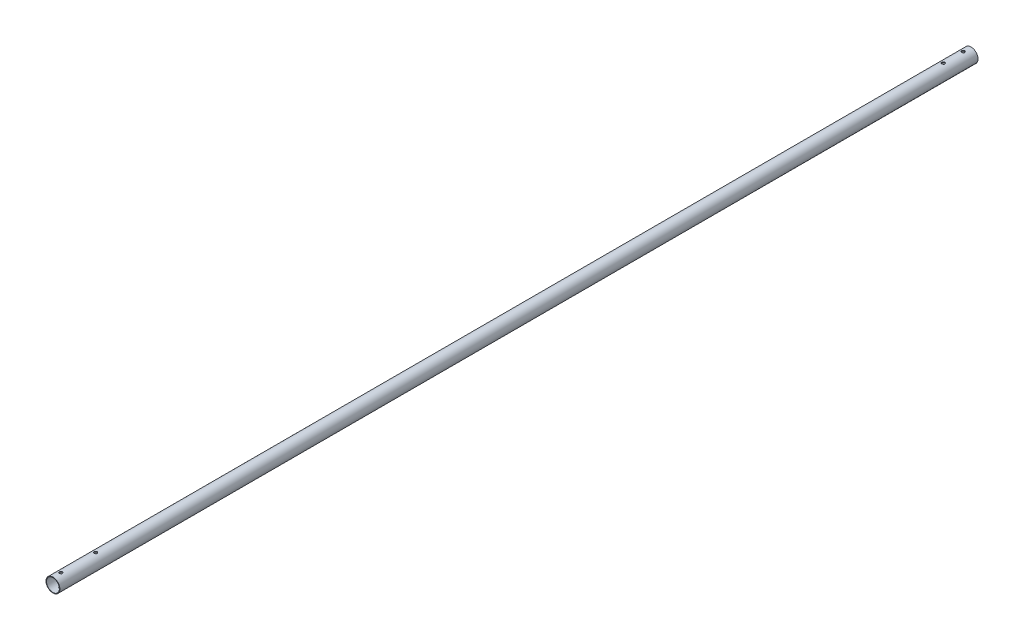
SolidWorks part; units mm, degrees
material "Thornel Mat VMA"
ref_plane "前视基准面" through (0, 0, 0) normal (0, 0, 1) x (1, 0, 0)
ref_plane "上视基准面" through (0, 0, 0) normal (0, 1, 0) x (1, 0, 0)
ref_plane "右视基准面" through (0, 0, 0) normal (1, 0, 0) x (0, 0, -1)
other "Configuration Table"
sketch "草图1" plane through (0, 0, 0) normal (0, 0, 1) x (1, 0, 0)
  circle A0 centre (0, 0) radius 7
  circle A1 centre (0, 0) radius 6.5
  dimension "D1" = 13
  dimension "D2" = 14
extrude "凸台-拉伸1" add sketch "草图1" against normal blind 926.63
sketch "草图2" plane through (0, 0, 0) normal (0, 1, 0) x (1, 0, 0)
  line L0 (0, 0) -> (0, 820.7577) construction
  line L1 (-7, 0) -> (7, 0) construction
  line L2 (7, 926.63) -> (-7, 926.63) construction
  circle A0 centre (0, 8) radius 1.55
  circle A1 centre (0, 43) radius 1.55
  circle A2 centre (0, 918.63) radius 1.55
  circle A3 centre (0, 898.63) radius 1.55
  point P15 (0, 0)
  point P16 (0, 0)
  dimension "D1" = 3.1
  dimension "D2" = 35
  dimension "D4" = 8
  dimension "D5" = 20
  dimension "D3" = 8
extrude "切除-拉伸1" cut sketch "草图2" against normal through all both and the other way through all
